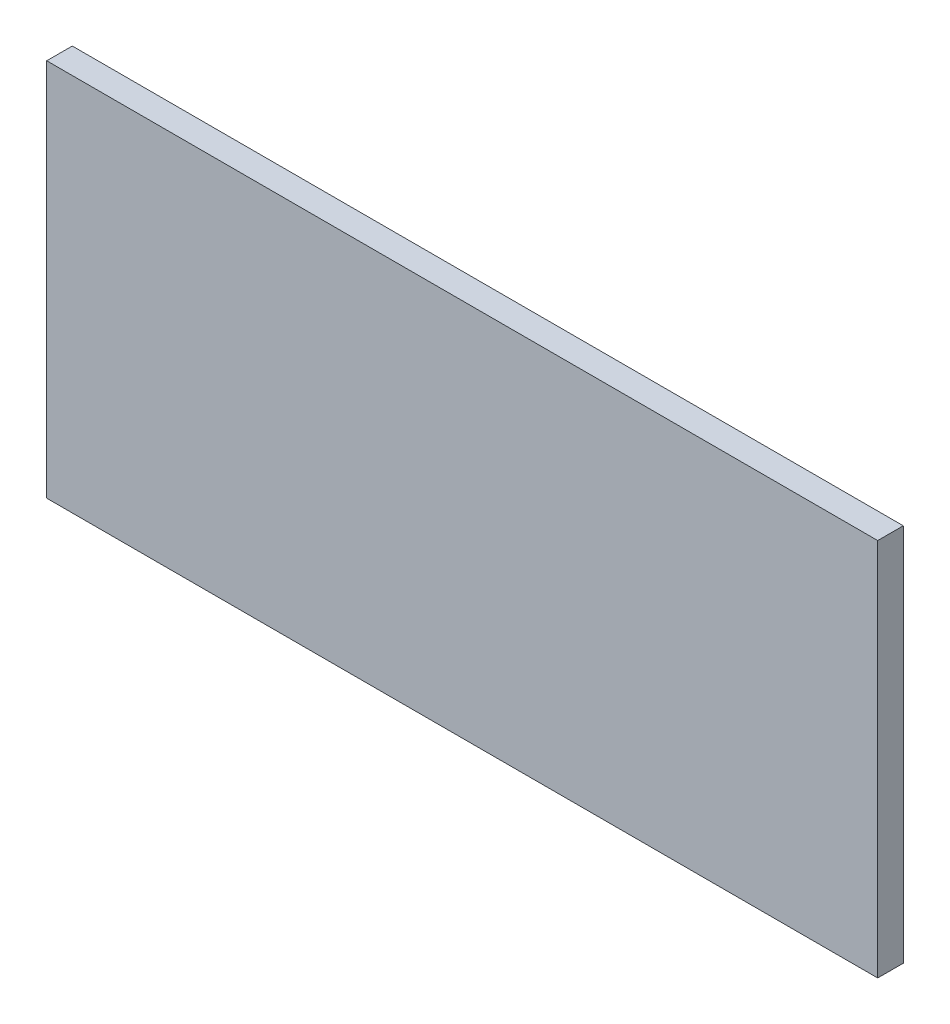
SolidWorks part; units mm, degrees
material "Q235B"
ref_plane "Front Plane" through (0, 0, 0) normal (0, 0, 1) x (1, 0, 0)
ref_plane "Top Plane" through (0, 0, 0) normal (0, 1, 0) x (1, 0, 0)
ref_plane "Right Plane" through (0, 0, 0) normal (1, 0, 0) x (0, 0, -1)
sketch "Sketch1" plane through (0, 0, 0) normal (0, 0, 1) x (1, 0, 0)
  line L0 (0, 77.8126) -> (0, -64.9863) construction
  line L1 (-195, 88.9) -> (195, 88.9)
  line L2 (-195, 88.9) -> (-195, -88.9)
  line L3 (-195, -88.9) -> (195, -88.9)
  line L4 (195, 88.9) -> (195, -88.9)
  line L5 (-120.6596, 0) -> (106.8741, 0) construction
  dimension "D1" = 390
  dimension "D2" = 177.8
extrude "Extrude1" add sketch "Sketch1" along normal mid plane 12
